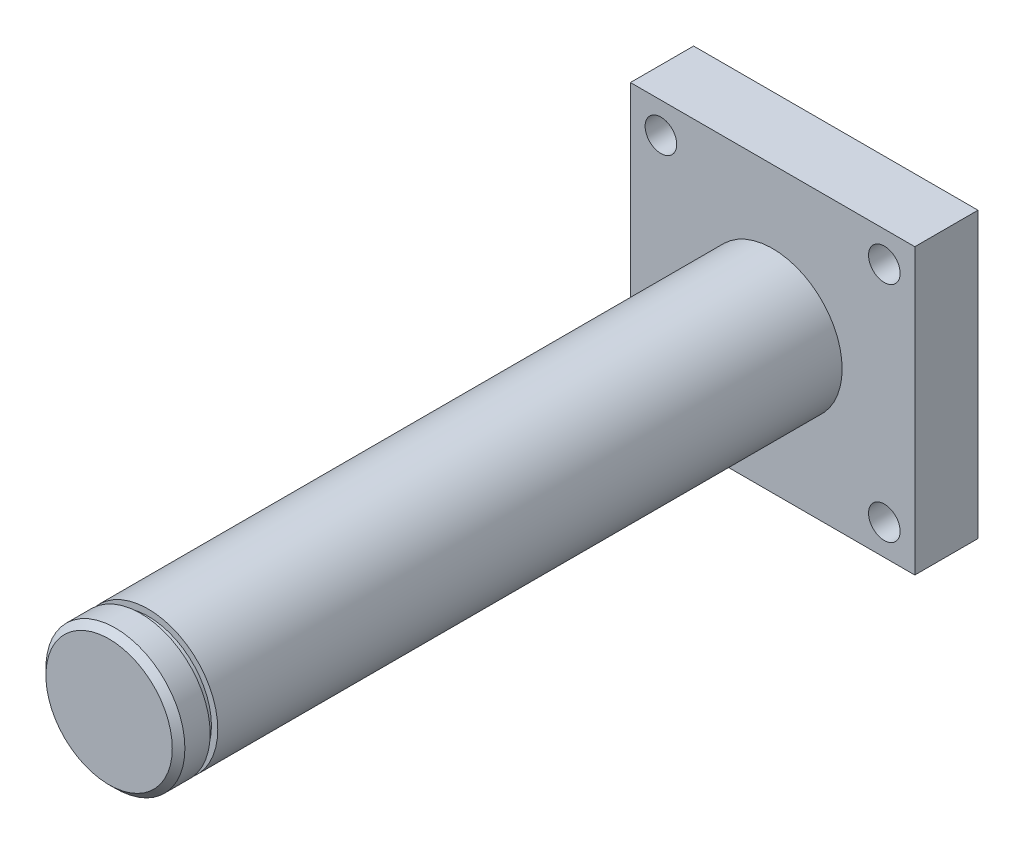
from build123d import *

# Parameters (mm, degrees)
SKETCH1_W           = 45
SKETCH1_H           = 45
SKETCH1_R           = 2.5
BOSS_EXTRUDE1_DEPTH = 10
SKETCH2_R           = 11
BOSS_EXTRUDE2_DEPTH = 105
CHAMFER1_SIZE       = 1
CUT_EXTRUDE1_START  = -5
SKETCH3_R           = 12.248377089
SKETCH3_R_2         = 10
CUT_EXTRUDE1_DEPTH  = 1.2


with BuildPart() as part:
    # Sketch1 → Boss-Extrude1 (new body)
    with BuildSketch(Plane.XY):
        Rectangle(SKETCH1_W, SKETCH1_H)
        with Locations((17.67766953, 17.67766953)):
            Circle(SKETCH1_R, mode=Mode.SUBTRACT)
        with Locations((17.67766953, -17.67766953)):
            Circle(SKETCH1_R, mode=Mode.SUBTRACT)
        with Locations((-17.67766953, -17.67766953)):
            Circle(SKETCH1_R, mode=Mode.SUBTRACT)
        with Locations((-17.67766953, 17.67766953)):
            Circle(SKETCH1_R, mode=Mode.SUBTRACT)
    extrude(amount=BOSS_EXTRUDE1_DEPTH)

    # Sketch2 → Boss-Extrude2 (add)
    with BuildSketch(Plane.XY.offset(10)):
        Circle(SKETCH2_R)
    extrude(amount=BOSS_EXTRUDE2_DEPTH)

    # Chamfer1
    chamfer1_edges = [part.edges().sort_by_distance(p)[0] for p in [
        (-11, 0, 115),
    ]]
    chamfer(chamfer1_edges, length=CHAMFER1_SIZE)

    # Sketch3 → Cut-Extrude1 (cut)
    with BuildSketch(Plane.XY.offset(115).offset(CUT_EXTRUDE1_START)):
        Circle(SKETCH3_R)
        Circle(SKETCH3_R_2, mode=Mode.SUBTRACT)
    extrude(amount=-CUT_EXTRUDE1_DEPTH, mode=Mode.SUBTRACT)


solid = part.part
